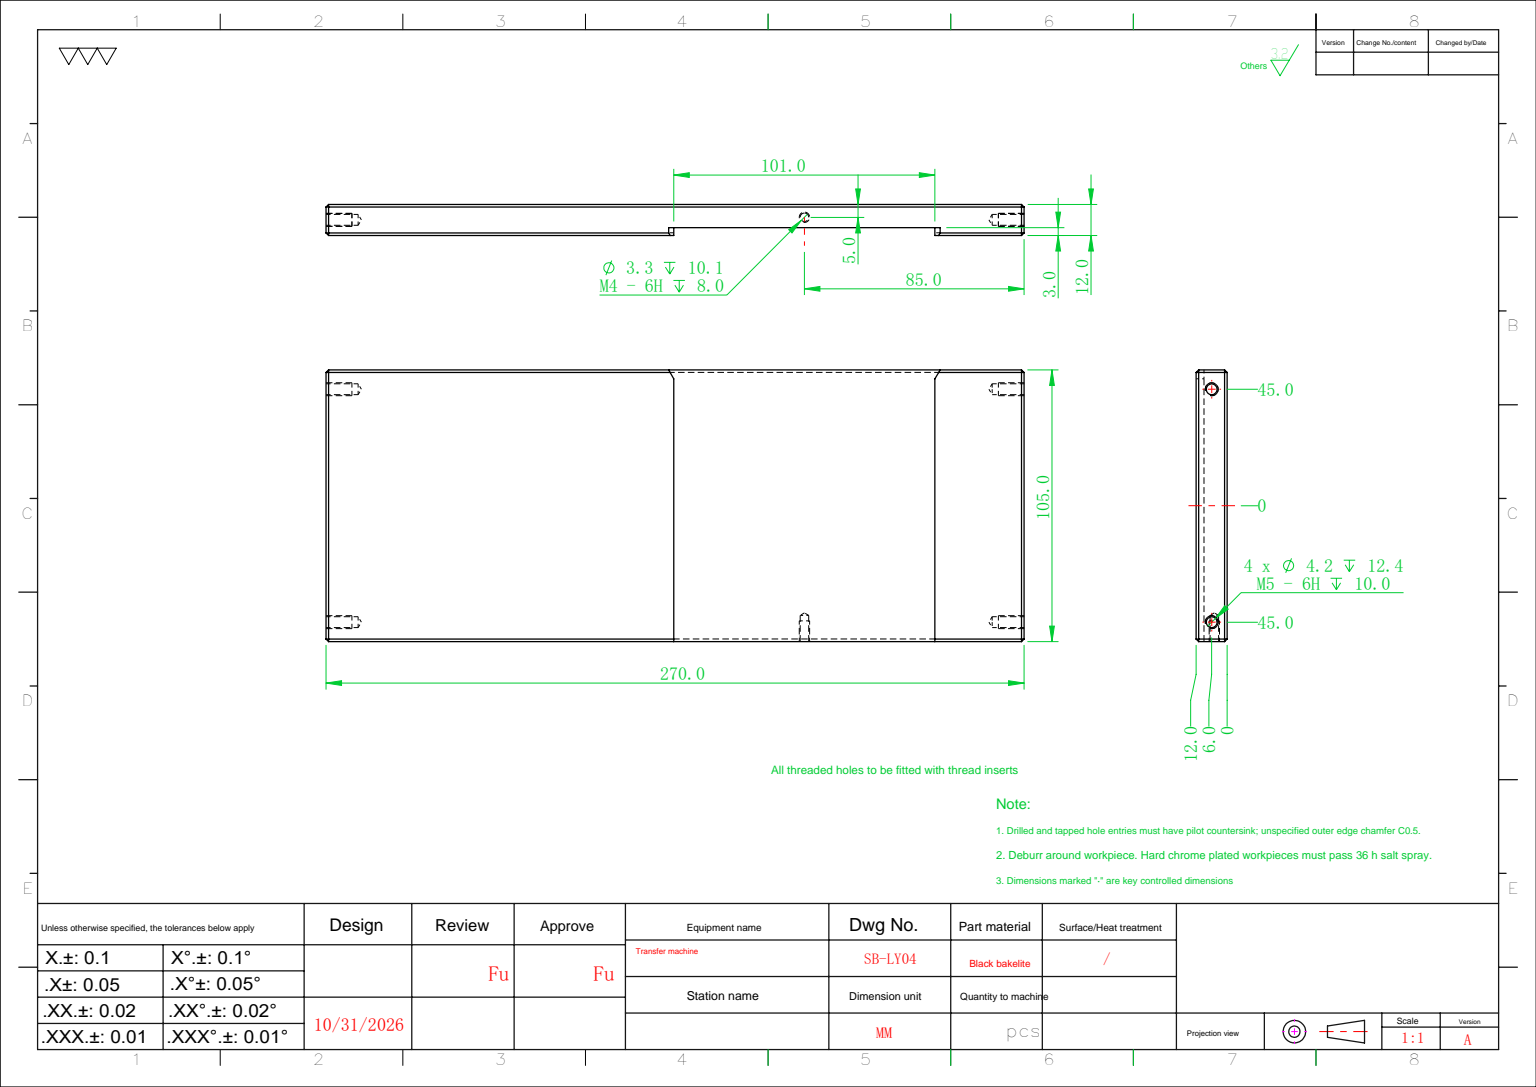
SolidWorks part; units mm, degrees
ref_plane "前视基准面" through (0, 0, 0) normal (0, 0, 1) x (1, 0, 0)
ref_plane "上视基准面" through (0, 0, 0) normal (0, 1, 0) x (1, 0, 0)
ref_plane "右视基准面" through (0, 0, 0) normal (1, 0, 0) x (0, 0, -1)
sketch "草图1" plane through (0, 0, 0) normal (0, 0, 1) x (1, 0, 0)
  line L1 (-52.5, -135) -> (52.5, -135)
  line L2 (-52.5, -135) -> (-52.5, 135)
  line L3 (-52.5, 135) -> (52.5, 135)
  line L4 (52.5, -135) -> (52.5, 135)
  line L5 (-52.5, -135) -> (52.5, 135) construction
  line L6 (-52.5, 135) -> (52.5, -135) construction
  point P0 (0, 0)
  dimension "D1" = 105
  dimension "D2" = 270
extrude "凸台-拉伸1" add sketch "草图1" along normal blind 12
sketch "草图2" plane through (52.5, 0, 0) normal (1, 0, 0) x (0, 0, -1)
  line L0 (-12, -135) -> (-12, 135) construction
  line L1 (-12, -0.5) -> (-9, -0.5)
  line L2 (-12, -0.5) -> (-12, 100.5)
  line L3 (-12, 100.5) -> (-9, 100.5)
  line L4 (-9, -0.5) -> (-9, 100.5)
  line L5 (-49, 50) -> (17.4235, 50) construction
  dimension "D1" = 50
  dimension "D2" = 101
  dimension "D3" = 3
extrude "切除-拉伸1" cut sketch "草图2" against normal through all
hole_wizard "M5 螺纹孔1" positions "草图3" profile "草图4" tap size "M5" standard "ISO"
sketch "草图3" plane through (0, -135, 0) normal (0, -1, 0) x (-1, 0, 0)
  line L0 (0, 0) -> (0, -12) construction
  line L1 (52.5, -12) -> (-52.5, -12) construction
  line L3 (52.5, -6) -> (-52.5, -6) construction
  line L4 (52.5, -12) -> (52.5, 0) construction
  line L5 (-52.5, -12) -> (-52.5, 0) construction
  point P0 (45, -6)
  point P2 (-45, -6)
  dimension "D1" = 90
sketch "草图4" plane through (-45, -135, 6) normal (1, 0, 0) x (0, 0, -1)
  line L0 (0, 0) -> (0, 13.6618)
  line L1 (0, 13.6618) -> (2.1, 12.4)
  line L2 (2.1, 12.4) -> (2.1, 0)
  line L5 (2.1, 0) -> (0, 0)
  line L10 (0, 13.6618) -> (-2.1, 12.4) construction
  line L11 (0, -6.35) -> (0, 107.95) construction
  dimension "螺纹孔钻头直径" = 4.2
  dimension "螺纹孔钻头深度" = 12.4
  dimension "导头角度" = 118
cosmetic thread "孔螺蚊线1" parameters "D1"=10, "D2"=5
cosmetic thread "孔螺蚊线2" parameters "D1"=10, "D2"=5
mirror "镜向1" about plane through (0, 0, 0) normal (0, 1, 0) of "M5 螺纹孔1"
chamfer "倒角1" distance 1 angle 45 14 edges at (52.5, 135, 6) (52.5, 117.75, 12) (0, 135, 12) (-52.5, 117.75, 12) (-52.5, 135, 6) (0, 135, 0) (-52.5, -135, 6) (-52.5, -67.75, 12) (0, -135, 12) (-52.5, 0, 0) (0, -135, 0) (52.5, 0, 0) (52.5, -135, 6) (52.5, -67.75, 12)
chamfer "倒角2" distance 2 angle 60 2 edges at (-52.5, -0.5, 10) (-52.5, 100.5, 10)
hole_wizard "M4 螺纹孔1" positions "草图5" profile "草图7" tap size "M4" standard "ISO"
sketch "草图5" plane through (52.5, 0, 0) normal (1, 0, 0) x (0, 0, -1)
  line L0 (-9, 50) -> (2.6546, 50) construction
  line L1 (-9, -0.5) -> (-9, 100.5) construction
  point P0 (-5, 50)
  dimension "D1" = 4
sketch "草图7" plane through (52.5, 50, 5) normal (0, 1, 0) x (0, 0, -1)
  line L0 (0, 0) -> (0, 11.0914)
  line L1 (0, 11.0914) -> (1.65, 10.1)
  line L2 (1.65, 10.1) -> (1.65, 0)
  line L5 (1.65, 0) -> (0, 0)
  line L10 (0, 11.0914) -> (-1.65, 10.1) construction
  line L11 (0, -6.35) -> (0, 107.95) construction
  dimension "螺纹孔钻头直径" = 3.3
  dimension "螺纹孔钻头深度" = 10.1
  dimension "导头角度" = 118
cosmetic thread "孔螺蚊线3" parameters "D1"=8, "D2"=4
